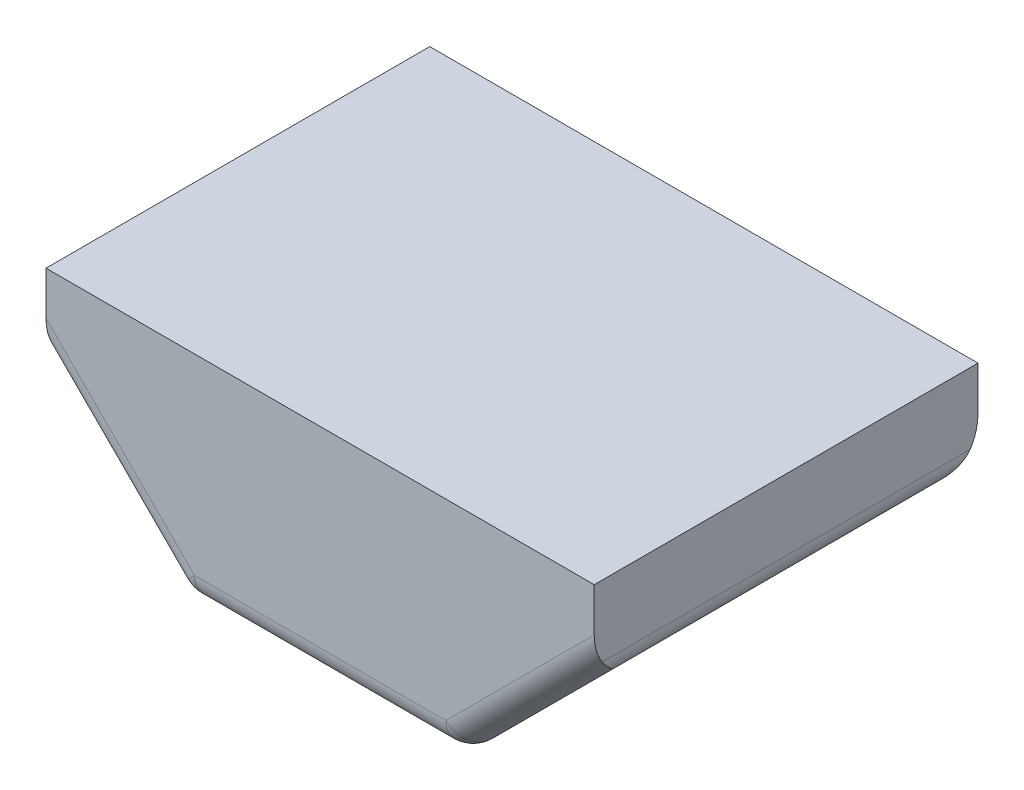
from build123d import *

# Parameters (mm, degrees)
EXTRUDE_1_DEPTH = 70
FILLET_1_R      = 5


with BuildPart() as part:
    # 草图1 → 凸台-拉伸1 (new body)
    with BuildSketch(Plane.XY):
        Polygon((0, 0), (100, 0), (100, -15), (75, -40), (50, -40), (25, -40), (0, -15), align=None)
    extrude(amount=EXTRUDE_1_DEPTH)

    # 圆角1
    fillet_1_edges = [part.edges().sort_by_distance(p)[0] for p in [
        (50, -40, 70),
        (100, -15, 35),
        (75, -40, 35),
        (25, -40, 35),
        (0, -15, 35),
        (87.5, -27.5, 70),
        (12.5, -27.5, 70),
        (87.5, -27.5, 0),
        (50, -40, 0),
        (12.5, -27.5, 0),
    ]]
    fillet(fillet_1_edges, radius=FILLET_1_R)


solid = part.part
